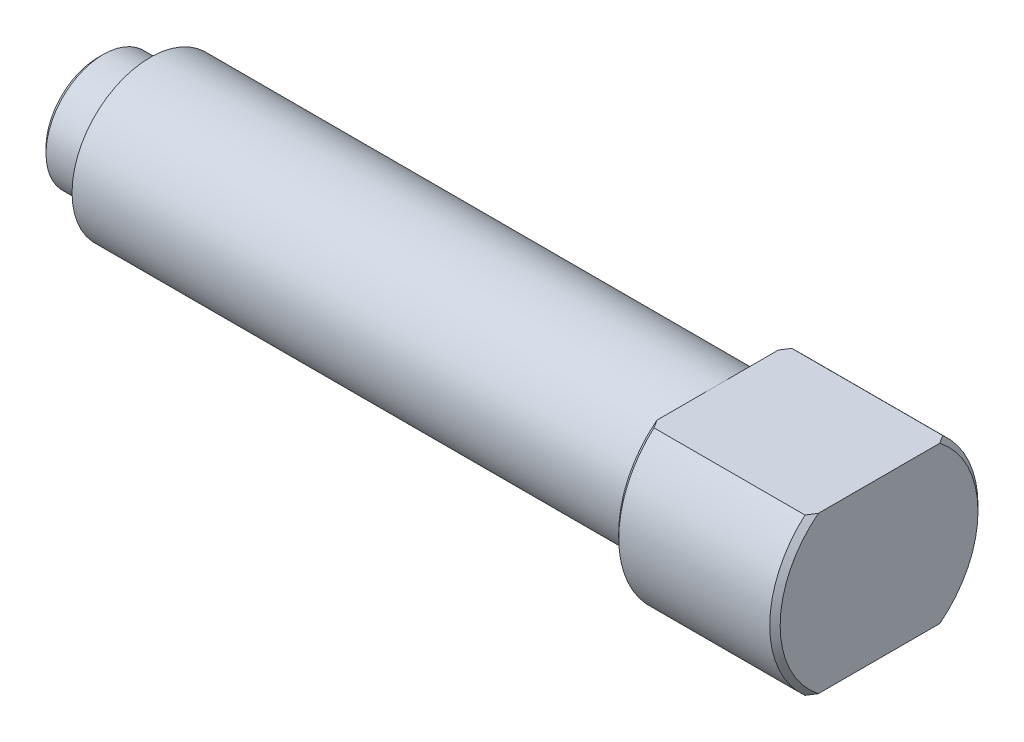
from build123d import *

# Parameters (mm, degrees)
SKETCH1_W             = 75
SKETCH1_H             = 7.5
CHAMFER3_SIZE         = 0.5
M6_TAPPED_HOLE1_D     = 5
M6_TAPPED_HOLE1_DEPTH = 15
M6_TAPPED_HOLE1_TIP   = 1.502151548
SKETCH7_R             = 10
BOSS_EXTRUDE2_DEPTH   = 15.5
CHAMFER4_SIZE         = 0.5
SKETCH8_OUTSIDE_W     = 38.032
SKETCH8_OUTSIDE_H     = 38.032
SKETCH8_OUTSIDE_W_2   = 25
SKETCH8_OUTSIDE_H_2   = 15
CUT_EXTRUDE1_DEPTH    = 62.15758334
SKETCH11_OUTSIDE_W    = 37.812
SKETCH11_OUTSIDE_H    = 32.812
SKETCH11_OUTSIDE_R    = 5.5
CUT_EXTRUDE2_DEPTH    = 5
CHAMFER5_SIZE         = 0.5


with BuildPart() as part:
    # Sketch1 → Revolve1 (revolve)
    with BuildSketch(Plane.XY, mode=Mode.PRIVATE) as revolve1_sk:
        with Locations((0, 3.75)):
            Rectangle(SKETCH1_W, SKETCH1_H)
    revolve(revolve1_sk.sketch.rotate(Axis((-37.5, 0, 0), (1, 0, 0)), 90), axis=Axis((-37.5, 0, 0), (1, 0, 0)))

    # Chamfer3
    chamfer3_edges = [part.edges().sort_by_distance(p)[0] for p in [
        (-37.5, 0, -7.5),
    ]]
    chamfer(chamfer3_edges, length=CHAMFER3_SIZE)

    # M6 Tapped Hole1
    with Locations(Plane.ZY.offset(37.5)):
        with Locations((0, 0)):
            Hole(M6_TAPPED_HOLE1_D / 2, depth=M6_TAPPED_HOLE1_DEPTH)
            with Locations((0, 0, -(M6_TAPPED_HOLE1_DEPTH + M6_TAPPED_HOLE1_TIP / 2))):  # 118° drill point
                Cone(0, M6_TAPPED_HOLE1_D / 2, M6_TAPPED_HOLE1_TIP, mode=Mode.SUBTRACT)

    # Sketch7 → Boss-Extrude2 (add)
    with BuildSketch(Plane(origin=(37.5, 0, 0), x_dir=(0, 0, -1), z_dir=(1, 0, 0))):
        Circle(SKETCH7_R)
    extrude(amount=-BOSS_EXTRUDE2_DEPTH)

    # Chamfer4
    chamfer4_edges = [part.edges().sort_by_distance(p)[0] for p in [
        (22, 0, 10),
        (37.5, 0, 10),
    ]]
    chamfer(chamfer4_edges, length=CHAMFER4_SIZE)

    # Sketch8 outside → Cut-Extrude1 (cut, through all)
    with BuildSketch(Plane.ZY.offset(-22)):
        Rectangle(SKETCH8_OUTSIDE_W, SKETCH8_OUTSIDE_H)
        Rectangle(SKETCH8_OUTSIDE_W_2, SKETCH8_OUTSIDE_H_2, mode=Mode.SUBTRACT)
    extrude(amount=-CUT_EXTRUDE1_DEPTH, mode=Mode.SUBTRACT)

    # Sketch11 outside → Cut-Extrude2 (cut)
    with BuildSketch(Plane.ZY.offset(37.5)):
        Rectangle(SKETCH11_OUTSIDE_W, SKETCH11_OUTSIDE_H)
        Circle(SKETCH11_OUTSIDE_R, mode=Mode.SUBTRACT)
    extrude(amount=-CUT_EXTRUDE2_DEPTH, mode=Mode.SUBTRACT)

    # Chamfer5
    chamfer5_edges = [part.edges().sort_by_distance(p)[0] for p in [
        (-37.5, 0, -5.5),
    ]]
    chamfer(chamfer5_edges, length=CHAMFER5_SIZE)


solid = part.part
